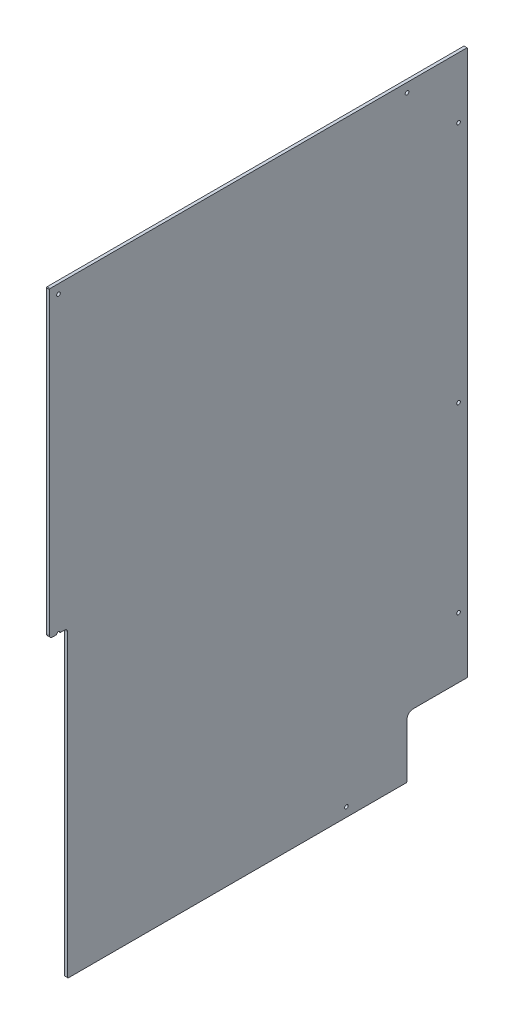
from build123d import *

# Parameters (mm, degrees)
SKETCH_1_W                = 690
SKETCH_1_H                = 1000
EXTRUDE_1_DEPTH           = 5
CHAMFER_1_SIZE            = 1
SKETCH_2_R                = 3
CUT_EXTRUDE_1_DEPTH       = 608.494855945
SKETCH_3_W                = 100
SKETCH_3_H                = 100
CUT_EXTRUDE_2_DEPTH       = 608.494855945
HOLE_WIZARD_6_0_6_1_D     = 6
HOLE_WIZARD_6_0_6_1_DEPTH = 5
HOLE_WIZARD_6_0_6_1_TIP   = 3
FILLET_1_R                = 10
SKETCH_6_W                = 30
SKETCH_6_H                = 500
CUT_EXTRUDE_3_DEPTH       = 10
CHAMFER_2_SIZE            = 1
FILLET_2_R                = 5


with BuildPart() as part:
    # 草图1 → 凸台-拉伸1 (new body)
    with BuildSketch(Plane(origin=(0, 0, 0), x_dir=(0, 0, -1), z_dir=(1, 0, 0))):
        Rectangle(SKETCH_1_W, SKETCH_1_H)
    extrude(amount=EXTRUDE_1_DEPTH)

    # 倒角1
    chamfer_1_edges = [part.edges().sort_by_distance(p)[0] for p in [
        (2.5, 500, 345),
        (2.5, 500, -345),
        (2.5, -500, -345),
        (2.5, -500, 345),
    ]]
    chamfer(chamfer_1_edges, length=CHAMFER_1_SIZE)

    # 草图2 → 切除-拉伸1 (cut, through all)
    with BuildSketch(Plane.ZY):
        with Locations(Location((-330, -485, 0), (0, 0, 180))):
            Circle(SKETCH_2_R)
        with Locations((330, -485)):
            Circle(SKETCH_2_R)
        with Locations(Location((330, 485, 0), (0, 0, 180))):
            Circle(SKETCH_2_R)
        with Locations((330, 0)):
            Circle(SKETCH_2_R)
        with Locations((-330, 0)):
            Circle(SKETCH_2_R)
    extrude(amount=-CUT_EXTRUDE_1_DEPTH, mode=Mode.SUBTRACT)

    # 草图3 → 切除-拉伸2 (cut, through all)
    with BuildSketch(Plane.ZY):
        with Locations((-295, -450)):
            Rectangle(SKETCH_3_W, SKETCH_3_H)
    extrude(amount=-CUT_EXTRUDE_2_DEPTH, mode=Mode.SUBTRACT)

    # Ø6.0 (6) 直径孔1
    with Locations(Plane(origin=(0, -600, 465), x_dir=(0, 0, 1), z_dir=(-1, 0, 0))):
        with Locations((-710, 1085), (-795, 1000), (-795, 300), (-610, 115)):
            Hole(HOLE_WIZARD_6_0_6_1_D / 2, depth=HOLE_WIZARD_6_0_6_1_DEPTH)
            with Locations((0, 0, -(HOLE_WIZARD_6_0_6_1_DEPTH + HOLE_WIZARD_6_0_6_1_TIP / 2))):  # 90° drill point
                Cone(0, HOLE_WIZARD_6_0_6_1_D / 2, HOLE_WIZARD_6_0_6_1_TIP, mode=Mode.SUBTRACT)

    # 圆角1
    fillet_1_edges = [part.edges().sort_by_distance(p)[0] for p in [
        (2.5, -400, -245),
    ]]
    fillet(fillet_1_edges, radius=FILLET_1_R)

    # 草图6 → 切除-拉伸3 (cut)
    with BuildSketch(Plane.ZY):
        with Locations((330, -250)):
            Rectangle(SKETCH_6_W, SKETCH_6_H)
    extrude(amount=-CUT_EXTRUDE_3_DEPTH, mode=Mode.SUBTRACT)

    # 倒角2
    chamfer_2_edges = [part.edges().sort_by_distance(p)[0] for p in [
        (2.5, -500, 315),
        (2.5, -500, -245),
        (2.5, -400, -345),
    ]]
    chamfer(chamfer_2_edges, length=CHAMFER_2_SIZE)

    # 圆角2
    fillet_2_edges = [part.edges().sort_by_distance(p)[0] for p in [
        (2.5, 0, 345),
        (2.5, 0, 315),
    ]]
    fillet(fillet_2_edges, radius=FILLET_2_R)


solid = part.part
